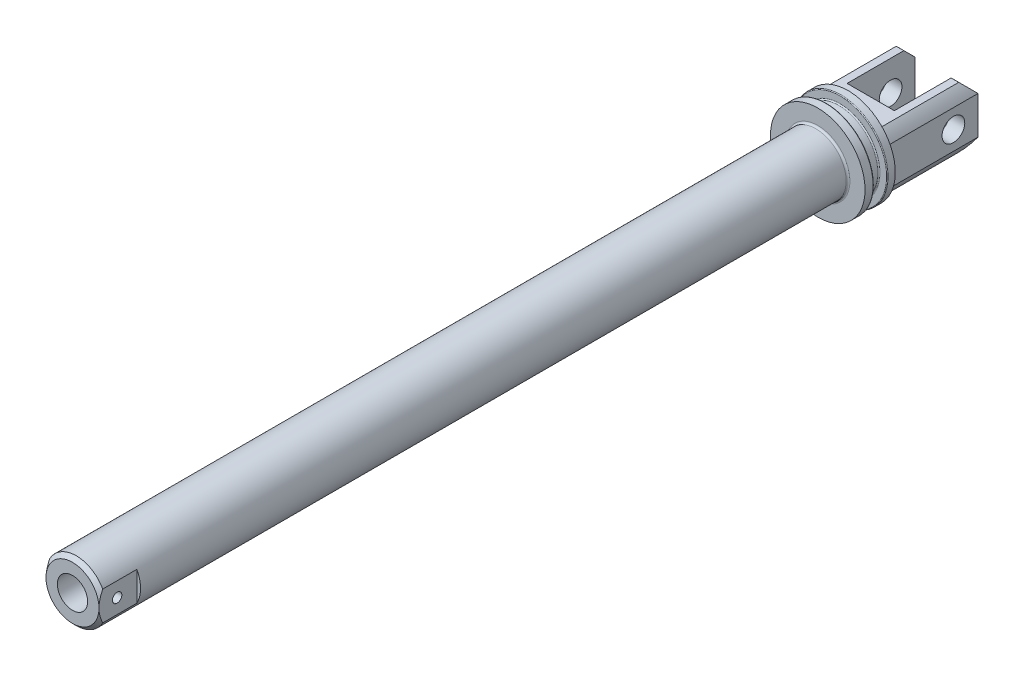
from build123d import *

# Parameters (mm, degrees)
SKETCH1_R               = 8
BOSS_EXTRUDE1_DEPTH     = 197
SKETCH2_R               = 12.5
BOSS_EXTRUDE2_DEPTH     = 8
SKETCH3_W               = 2.25
SKETCH3_H               = 3.6
SKETCH8_R               = 11.5
BOSS_EXTRUDE4_DEPTH     = 24
CUT_EXTRUDE1_DEPTH      = 198.791556948
CUT_EXTRUDE1_DEPTH_BACK = 198.791556948
SKETCH10_W              = 12.5
SKETCH10_H              = 21.605782088
CUT_EXTRUDE3_DEPTH      = 231.593256623
CUT_EXTRUDE3_DEPTH_BACK = 231.593256623
CUT_EXTRUDE5_START      = -24
CUT_EXTRUDE5_DEPTH      = 24
FILLET1_R               = 0.5
FILLET2_R               = 0.2
FILLET3_R               = 0.3
CHAMFER3_SIZE           = 1
CUT_EXTRUDE7_DEPTH      = 199.457804086
CUT_EXTRUDE7_DEPTH_BACK = 199.457804086
SKETCH15_W              = 2.199256875
SKETCH15_H              = 10
SKETCH15_W_2            = 2.880068719
SKETCH14_R              = 3
CUT_EXTRUDE6_DEPTH      = 24
HOLE2_D                 = 8
HOLE2_DEPTH             = 7.5
M6_TAPPED_HOLE1_D       = 5
M6_TAPPED_HOLE1_DEPTH   = 18
M6_TAPPED_HOLE1_TIP     = 1.502151548
M3_TAPPED_HOLE1_D       = 2.5
M3_TAPPED_HOLE1_DEPTH   = 7.5
M3_TAPPED_HOLE1_TIP     = 0.751075774


with BuildPart() as part:
    # Sketch1 → Boss-Extrude1 (new body)
    with BuildSketch(Plane.XY):
        Circle(SKETCH1_R)
    extrude(amount=BOSS_EXTRUDE1_DEPTH)

    # Sketch2 → Boss-Extrude2 (add)
    with BuildSketch(Plane(origin=(0, 0, 0), x_dir=(-1, 0, 0), z_dir=(0, 0, -1))):
        Circle(SKETCH2_R)
    extrude(amount=BOSS_EXTRUDE2_DEPTH)

    # Sketch3 → Cut-Revolve1 (revolve, cut)
    with BuildSketch(Plane(origin=(0, 0, 0), x_dir=(1, 0, 0), z_dir=(0, 1, 0))):
        with Locations((-11.375, 4.1)):
            Rectangle(SKETCH3_W, SKETCH3_H)
    revolve(axis=Axis((0, 0, -10.00817261), (0, 0, 1)), mode=Mode.SUBTRACT)

    # Sketch8 → Boss-Extrude4 (add)
    with BuildSketch(Plane(origin=(0, 0, -8), x_dir=(-1, 0, 0), z_dir=(0, 0, -1))):
        Circle(SKETCH8_R)
    extrude(amount=BOSS_EXTRUDE4_DEPTH)

    # Sketch10 → Cut-Extrude1 (cut, two sides: drawn at the far end of the back side and taken through both)
    with BuildSketch(Plane(origin=(0, 0, 0), x_dir=(1, 0, 0), z_dir=(0, 1, 0)).offset(-CUT_EXTRUDE1_DEPTH_BACK)):
        with Locations((0, 24.802891044)):
            Rectangle(SKETCH10_W, SKETCH10_H)
    extrude(amount=CUT_EXTRUDE1_DEPTH + CUT_EXTRUDE1_DEPTH_BACK, mode=Mode.SUBTRACT)

    # Sketch11 → Cut-Extrude3 (cut, two sides: drawn at the far end of the back side and taken through both)
    with BuildSketch(Plane(origin=(0, -11.5, -32), x_dir=(0, 0, -1), z_dir=(-1, 0, 0)).offset(-CUT_EXTRUDE3_DEPTH_BACK)):
        Polygon((0.010981051, -16.5), (-3, -19.5), (-24, -19.5), (-24, -26.396557876), (1.498378991, -26.396557876), (1.498378991, -19.5), (0.010981051, -19.5), align=None)
        Polygon((-24, -3.5), (-24, 3.359688932), (2.769529036, 3.359688932), (2.769529036, -3.5), (1.498378991, -3.5), (0.010981051, -3.5), (0.010981051, -6.5), (-3, -3.5), align=None)
    extrude(amount=CUT_EXTRUDE3_DEPTH + CUT_EXTRUDE3_DEPTH_BACK, mode=Mode.SUBTRACT)

    # Sketch13 → Cut-Extrude5 (cut)
    with BuildSketch(Plane(origin=(0, 0, -32), x_dir=(-1, 0, 0), z_dir=(0, 0, -1)).offset(CUT_EXTRUDE5_START)):
        with BuildLine():
            Line((10.356157589, -5), (10.356157589, 5))
            ThreePointArc((10.356157589, 5), (11.5, 0), (10.356157589, -5))
        make_face()
        with BuildLine():
            Line((-10.356157589, -5), (-10.356157589, 5))
            ThreePointArc((-10.356157589, 5), (-11.5, 0), (-10.356157589, -5))
        make_face()
    extrude(amount=CUT_EXTRUDE5_DEPTH, mode=Mode.SUBTRACT)

    # Fillet1
    fillet1_edges = [part.edges().sort_by_distance(p)[0] for p in [
        (-8, 0, 0),
    ]]
    fillet(fillet1_edges, radius=FILLET1_R)

    # Fillet2
    fillet2_edges = [part.edges().sort_by_distance(p)[0] for p in [
        (12.5, 0, -2.3),
        (12.5, 0, -5.9),
    ]]
    fillet(fillet2_edges, radius=FILLET2_R)

    # Fillet3
    fillet3_edges = [part.edges().sort_by_distance(p)[0] for p in [
        (10.25, 0, -2.3),
        (10.25, 0, -5.9),
    ]]
    fillet(fillet3_edges, radius=FILLET3_R)

    # Chamfer3
    chamfer3_edges = [part.edges().sort_by_distance(p)[0] for p in [
        (-8, 0, 197),
    ]]
    chamfer(chamfer3_edges, length=CHAMFER3_SIZE)

    # Sketch15 → Cut-Extrude7 (cut, two sides: drawn at the far end of the back side and taken through both)
    with BuildSketch(Plane(origin=(0, 8, 0), x_dir=(1, 0, 0), z_dir=(0, 1, 0)).offset(-CUT_EXTRUDE7_DEPTH_BACK)):
        with Locations((-8.099628438, -192)):
            Rectangle(SKETCH15_W, SKETCH15_H)
        with BuildLine():
            Line((-8.5, -153.05), (-9.470215056, -153.05))
            Line((-9.470215056, -153.05), (-9.470215056, -177.95))
            Line((-9.470215056, -177.95), (-8.5, -177.95))
            ThreePointArc((-8.5, -177.95), (-6.732233047, -177.217766953), (-6, -175.45))
            Line((-6, -175.45), (-6, -155.55))
            ThreePointArc((-6, -155.55), (-6.732233047, -153.782233047), (-8.5, -153.05))
        make_face()
        with Locations((8.44003436, -192)):
            Rectangle(SKETCH15_W_2, SKETCH15_H)
    extrude(amount=CUT_EXTRUDE7_DEPTH + CUT_EXTRUDE7_DEPTH_BACK, mode=Mode.SUBTRACT)

    # Sketch14 → Cut-Extrude6 (cut)
    with BuildSketch(Plane(origin=(10.356157589, 0, 0), x_dir=(0, 0, -1), z_dir=(1, 0, 0))):
        with Locations(Location((25.5, 0, 0), (0, 0, 90))):
            Circle(SKETCH14_R)
    extrude(amount=-CUT_EXTRUDE6_DEPTH, mode=Mode.SUBTRACT)

    # Hole2
    with Locations(Plane.XY.offset(197)):
        with Locations((0, 0)):
            Hole(HOLE2_D / 2, depth=HOLE2_DEPTH)

    # M6 Tapped Hole1
    with Locations(Plane.XY.offset(197)):
        with Locations((0, 0)):
            Hole(M6_TAPPED_HOLE1_D / 2, depth=M6_TAPPED_HOLE1_DEPTH)
            with Locations((0, 0, -(M6_TAPPED_HOLE1_DEPTH + M6_TAPPED_HOLE1_TIP / 2))):  # 118° drill point
                Cone(0, M6_TAPPED_HOLE1_D / 2, M6_TAPPED_HOLE1_TIP, mode=Mode.SUBTRACT)

    # M3 Tapped Hole1
    with Locations(Plane(origin=(7, 0, 0), x_dir=(0, 0, -1), z_dir=(1, 0, 0))):
        with Locations((-192.2, 0)):
            Hole(M3_TAPPED_HOLE1_D / 2, depth=M3_TAPPED_HOLE1_DEPTH)
            with Locations((0, 0, -(M3_TAPPED_HOLE1_DEPTH + M3_TAPPED_HOLE1_TIP / 2))):  # 118° drill point
                Cone(0, M3_TAPPED_HOLE1_D / 2, M3_TAPPED_HOLE1_TIP, mode=Mode.SUBTRACT)


solid = part.part
